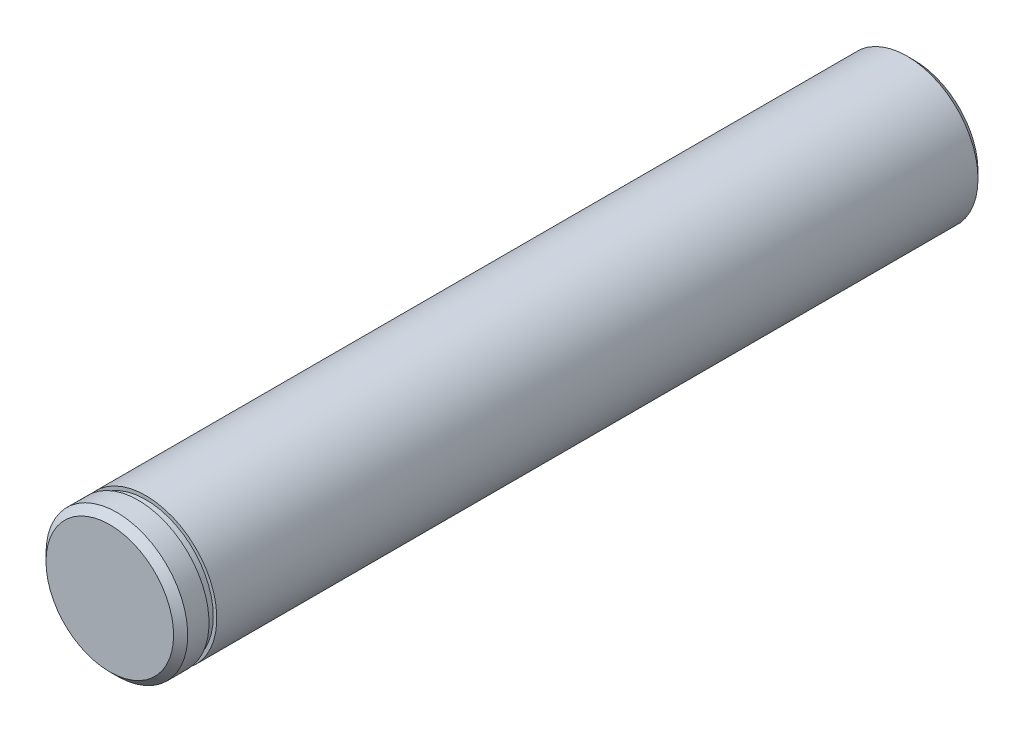
SolidWorks part; units mm, degrees
material "SUS304"
ref_plane "前视基准面" through (0, 0, 0) normal (0, 0, 1) x (1, 0, 0)
ref_plane "上视基准面" through (0, 0, 0) normal (0, 1, 0) x (1, 0, 0)
ref_plane "右视基准面" through (0, 0, 0) normal (1, 0, 0) x (0, 0, -1)
sketch "草图1" plane through (0, 0, 0) normal (0, 0, 1) x (1, 0, 0)
  circle A0 centre (0, 0) radius 10
  dimension "D1" = 20
extrude "凸台-拉伸1" add sketch "草图1" along normal blind 113.5
sketch "草图2" plane through (0, 0, 0) normal (0, 1, 0) x (1, 0, 0)
  line L0 (10, -113.5) -> (10, 0) construction
  line L1 (10, -108.4) -> (9.5, -108.4)
  line L2 (10, -108.4) -> (10, -109.5)
  line L3 (10, -109.5) -> (9.5, -109.5)
  line L4 (9.5, -108.4) -> (9.5, -109.5)
  line L5 (-10, -113.5) -> (10, -113.5) construction
  line L6 (0, -113.5) -> (0, -101.6093) construction
  dimension "D1" = 0.5
  dimension "D2" = 1.1
  dimension "D3" = 4
revolve "切除-旋转1" cut sketch "草图2" angle 360 about L6
chamfer "倒角1" distance 1 angle 45 2 edges at (10, 0, 0) (10, 0, 113.5)
hole_wizard "M6 螺纹孔1" positions "草图3" profile "草图4" tap size "M6" standard "ISO"
sketch "草图3" plane through (0, 0, 0) normal (0, 0, -1) x (-1, 0, 0)
  point P0 (0, 0)
sketch "草图4" plane through (0, 0, 0) normal (1, 0, 0) x (0, 1, 0)
  line L0 (0, 0) -> (0, 21)
  line L1 (0, 21) -> (2.5, 21)
  line L2 (2.5, 21) -> (2.5, 0)
  line L5 (2.5, 0) -> (0, 0)
  line L10 (0, 21) -> (-2.5, 21) construction
  line L11 (0, -6.35) -> (0, 107.95) construction
  dimension "螺纹孔钻头直径" = 5
  dimension "螺纹孔钻头深度" = 21
  dimension "导头角度" = 180
cosmetic thread "孔螺蚊线1" parameters "D1"=16, "D2"=6
